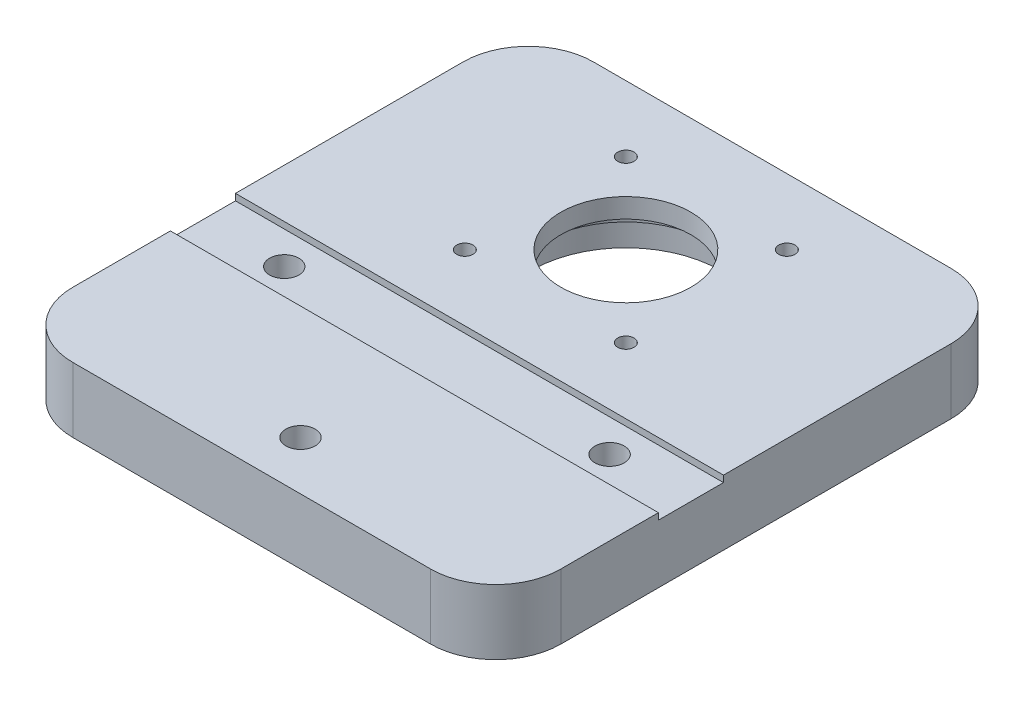
from build123d import *

# Parameters (mm, degrees)
SKETCH1_W                                           = 150
SKETCH1_H                                           = 160
BOSS_EXTRUDE1_DEPTH                                 = 20
SKETCH2_R                                           = 26
CUT_EXTRUDE1_DEPTH                                  = 14
SKETCH3_R                                           = 20
CUT_EXTRUDE2_DEPTH                                  = 14
M6_TAPPED_HOLE1_D                                   = 5
SKETCH9_R                                           = 29
CUT_EXTRUDE4_DEPTH                                  = 9
FILLET1_R                                           = 20
SKETCH10_W                                          = 150
SKETCH10_H                                          = 20
CUT_EXTRUDE5_DEPTH                                  = 2
HOLE_SIZE_BY_SOCKET_HEAD_CAP_SCREW_TYPE_D           = 9
HOLE_SIZE_BY_SOCKET_HEAD_CAP_SCREW_TYPE_CBORE_D     = 15
HOLE_SIZE_BY_SOCKET_HEAD_CAP_SCREW_TYPE_CBORE_DEPTH = 9


with BuildPart() as part:
    # Sketch1 → Boss-Extrude1 (new body)
    with BuildSketch(Plane.XZ):
        with Locations((75, -80)):
            Rectangle(SKETCH1_W, SKETCH1_H)
    extrude(amount=BOSS_EXTRUDE1_DEPTH)

    # Sketch2 → Cut-Extrude1 (cut)
    with BuildSketch(Plane.XZ.offset(20)):
        with Locations(Location((75, -115, 0), (0, 0, 270))):
            Circle(SKETCH2_R)
    extrude(amount=-CUT_EXTRUDE1_DEPTH, mode=Mode.SUBTRACT)

    # Sketch3 → Cut-Extrude2 (cut)
    with BuildSketch(Plane.XZ.offset(6)):
        with Locations(Location((75, -115, 0), (0, 0, 270))):
            Circle(SKETCH3_R)
    extrude(amount=-CUT_EXTRUDE2_DEPTH, mode=Mode.SUBTRACT)

    # M6 Tapped Hole1 (through all)
    with Locations(Plane(origin=(0, -20, 0), x_dir=(-1, 0, 0), z_dir=(0, -1, 0))):
        with Locations((-99.748737342, 139.748737342), (-50.251262658, 139.748737342), (-50.251262658, 90.251262658), (-99.748737342, 90.251262658)):
            Hole(M6_TAPPED_HOLE1_D / 2)

    # Sketch9 → Cut-Extrude4 (cut)
    with BuildSketch(Plane.XZ.offset(20)):
        with Locations(Location((75, -115, 0), (0, 0, 270))):
            Circle(SKETCH9_R)
    extrude(amount=-CUT_EXTRUDE4_DEPTH, mode=Mode.SUBTRACT)

    # Fillet1
    fillet1_edges = [part.edges().sort_by_distance(p)[0] for p in [
        (0, -10, 0),
        (150, -10, 0),
        (150, -10, -160),
        (0, -10, -160),
    ]]
    fillet(fillet1_edges, radius=FILLET1_R)

    # Sketch10 → Cut-Extrude5 (cut)
    with BuildSketch(Plane(origin=(0, 0, 0), x_dir=(1, 0, 0), z_dir=(0, 1, 0))):
        with Locations((75, 60)):
            Rectangle(SKETCH10_W, SKETCH10_H)
    extrude(amount=-CUT_EXTRUDE5_DEPTH, mode=Mode.SUBTRACT)

    # Hole size (by socket head cap screw type)1 (through all)
    with Locations(Plane(origin=(0, -20, 0), x_dir=(-1, 0, 0), z_dir=(0, -1, 0))):
        with Locations((-125, 60), (-25, 60), (-75, 15)):
            CounterBoreHole(HOLE_SIZE_BY_SOCKET_HEAD_CAP_SCREW_TYPE_D / 2, HOLE_SIZE_BY_SOCKET_HEAD_CAP_SCREW_TYPE_CBORE_D / 2, HOLE_SIZE_BY_SOCKET_HEAD_CAP_SCREW_TYPE_CBORE_DEPTH)


solid = part.part
